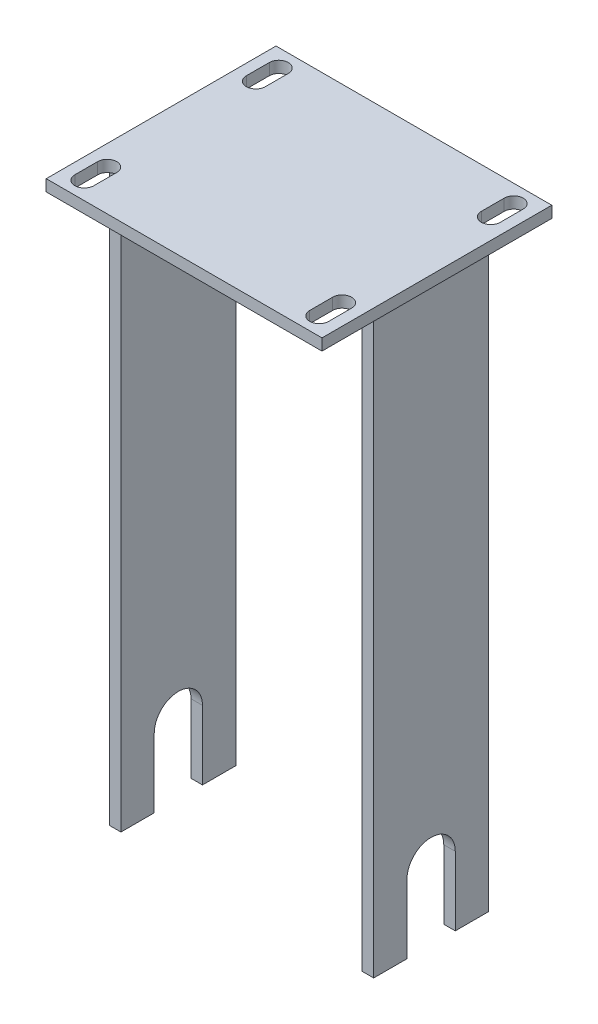
SolidWorks part; units mm, degrees
ref_plane "Front Plane" through (0, 0, 0) normal (0, 0, 1) x (1, 0, 0)
ref_plane "Top Plane" through (0, 0, 0) normal (0, 1, 0) x (1, 0, 0)
ref_plane "Right Plane" through (0, 0, 0) normal (1, 0, 0) x (0, 0, -1)
sketch "Sketch1" plane through (0, 0, 0) normal (0, 1, 0) x (1, 0, 0)
  line L1 (0, 0) -> (120, 0)
  line L2 (0, 0) -> (0, 100)
  line L3 (0, 100) -> (120, 100)
  line L4 (120, 0) -> (120, 100)
  dimension "D1" = 120
  dimension "D2" = 100
extrude "Boss-Extrude1" add sketch "Sketch1" along normal blind 5
sketch "Sketch2" plane through (0, 5, 0) normal (0, 1, 0) x (1, 0, 0)
  line L0 (8.8838, 92.3204) -> (8.8838, 82.3424) construction
  line L1 (13.0127, 92.3204) -> (13.0127, 82.3424)
  line L2 (4.755, 92.3204) -> (4.755, 82.3424)
  line L3 (0, 50) -> (120, 50) construction
  line L4 (0, 100) -> (0, 0) construction
  line L5 (120, 0) -> (120, 100) construction
  line L6 (60, 100) -> (60, 0) construction
  line L7 (120, 100) -> (0, 100) construction
  line L8 (0, 0) -> (120, 0) construction
  arc A0 (13.0127, 92.3204) -> (4.755, 92.3204) centre (8.8838, 92.3204) ccw
  arc A1 (4.755, 82.3424) -> (13.0127, 82.3424) centre (8.8838, 82.3424) ccw
  point P2 (8.8838, 87.3314)
extrude "Cut-Extrude1" cut sketch "Sketch2" against normal through all
sketch "Sketch3" plane through (0, 5, 0) normal (0, 1, 0) x (1, 0, 0)
  line L0 (60, 100) -> (60, 0) construction
  line L1 (120, 100) -> (0, 100) construction
  line L2 (0, 0) -> (120, 0) construction
  line L3 (0, 50) -> (120, 50) construction
  line L4 (0, 100) -> (0, 0) construction
  line L5 (120, 0) -> (120, 100) construction
ref_plane "Plane1" through (60, 0, 0) normal (-1, 0, 0) x (0, 0, 1)
mirror "Mirror1" about plane through (60, 0, 0) normal (-1, 0, 0) of "Cut-Extrude1"
ref_plane "Plane2" through (0, 0, -50) normal (0, 0, 1) x (1, 0, 0)
mirror "Mirror2" about plane through (0, 0, -50) normal (0, 0, 1) of "Mirror1", "Cut-Extrude1"
sketch "Sketch4" plane through (0, 0, 0) normal (0, -1, 0) x (1, 0, 0)
  line L3 (2.5, -50) -> (2.5, -75)
  line L4 (2.5, -50) -> (2.5, -25)
  line L5 (2.5, -25) -> (7.5, -25)
  line L7 (7.5, -50) -> (7.5, -25)
  line L8 (7.5, -50) -> (7.5, -75)
  line L9 (112.5, -75) -> (117.5, -75)
  line L10 (7.5, -75) -> (2.5, -75)
  line L11 (112.5, -45) -> (112.5, -75)
  line L13 (112.5, -45) -> (112.5, -25)
  line L14 (0, -50) -> (120, -50) construction
  line L16 (117.5, -25) -> (112.5, -25)
  line L17 (117.5, -45) -> (117.5, -25)
  line L18 (117.5, -45) -> (117.5, -75)
  dimension "D2" = 5
  dimension "D4" = 25
  dimension "D3" = 25
extrude "Boss-Extrude2" add sketch "Sketch4" along normal blind 250
sketch "Sketch5" plane through (2.5, 0, 0) normal (-1, 0, 0) x (0, 0, 1)
  line L0 (-25, -250) -> (-75, -250) construction
  line L1 (-50, -250) -> (-50, -220) construction
  line L2 (-60.5, -250) -> (-60.5, -220)
  line L3 (-39.5, -250) -> (-39.5, -220)
  arc A1 (-60.5, -250) -> (-39.5, -250) centre (-50, -250) ccw
  arc A2 (-39.5, -220) -> (-60.5, -220) centre (-50, -220) ccw
  point P4 (-50, -235)
  dimension "D1" = 30
extrude "Cut-Extrude2" cut sketch "Sketch5" against normal blind 450
